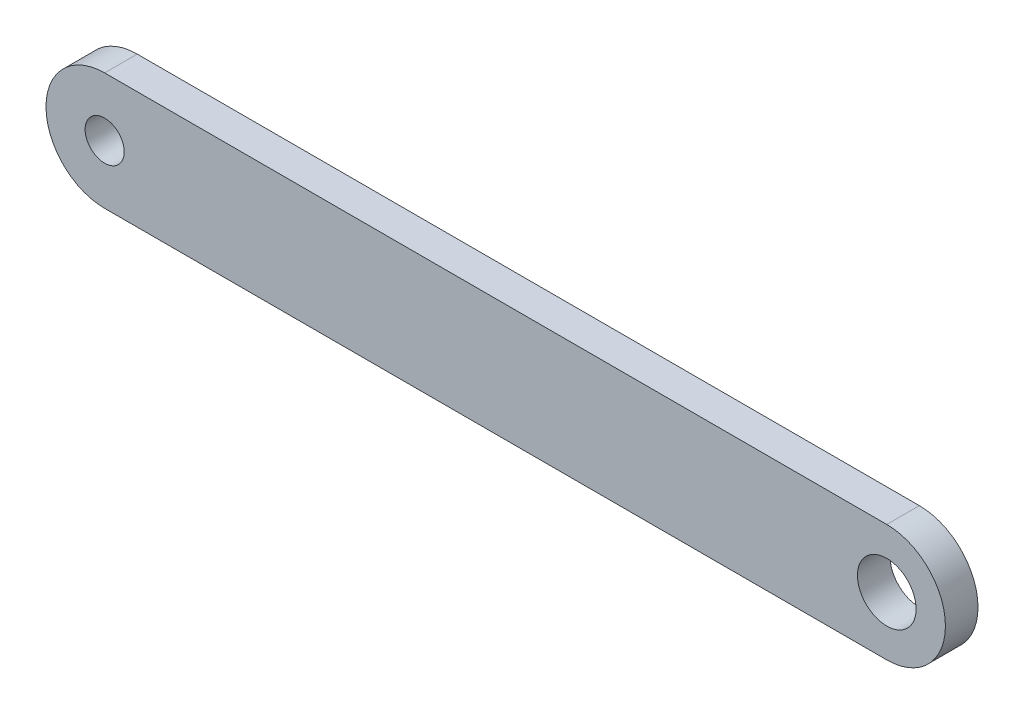
SolidWorks part; units mm, degrees
ref_plane "前视基准面" through (0, 0, 0) normal (0, 0, 1) x (1, 0, 0)
ref_plane "上视基准面" through (0, 0, 0) normal (0, 1, 0) x (1, 0, 0)
ref_plane "右视基准面" through (0, 0, 0) normal (1, 0, 0) x (0, 0, -1)
sketch "草图1" plane through (0, 0, 0) normal (0, 0, 1) x (1, 0, 0)
  line L0 (0, 0) -> (411.2456, 0) construction
  line L1 (0, 0) -> (120, 0) construction
  line L2 (0, 9) -> (120, 9)
  line L3 (0, -9) -> (120, -9)
  circle A0 centre (0, 0) radius 3
  circle A1 centre (120, 0) radius 3
  arc A2 (0, 9) -> (0, -9) centre (0, 0) ccw
  arc A3 (120, -9) -> (120, 9) centre (120, 0) ccw
  point P6 (60, 0)
  dimension "D1" = 120
  dimension "D2" = 6
  dimension "D3" = 6
  dimension "D4" = 9
extrude "凸台-拉伸1" add sketch "草图1" along normal blind 5
sketch "草图3" plane through (0, 0, 5) normal (0, 0, 1) x (1, 0, 0)
  circle A0 centre (120, 0) radius 6
extrude "切除-拉伸1" cut sketch "草图3" against normal blind 10
sketch "草图4" plane through (0, 0, 5) normal (0, 0, 1) x (1, 0, 0)
  circle A0 centre (120, 0) radius 4.5
  circle A1 centre (120, 0) radius 9
  dimension "D1" = 9
  dimension "D2" = 18
extrude "凸台-拉伸3" add sketch "草图4" against normal up to surface (5 mm away) up to face at (126, 0, 0)
